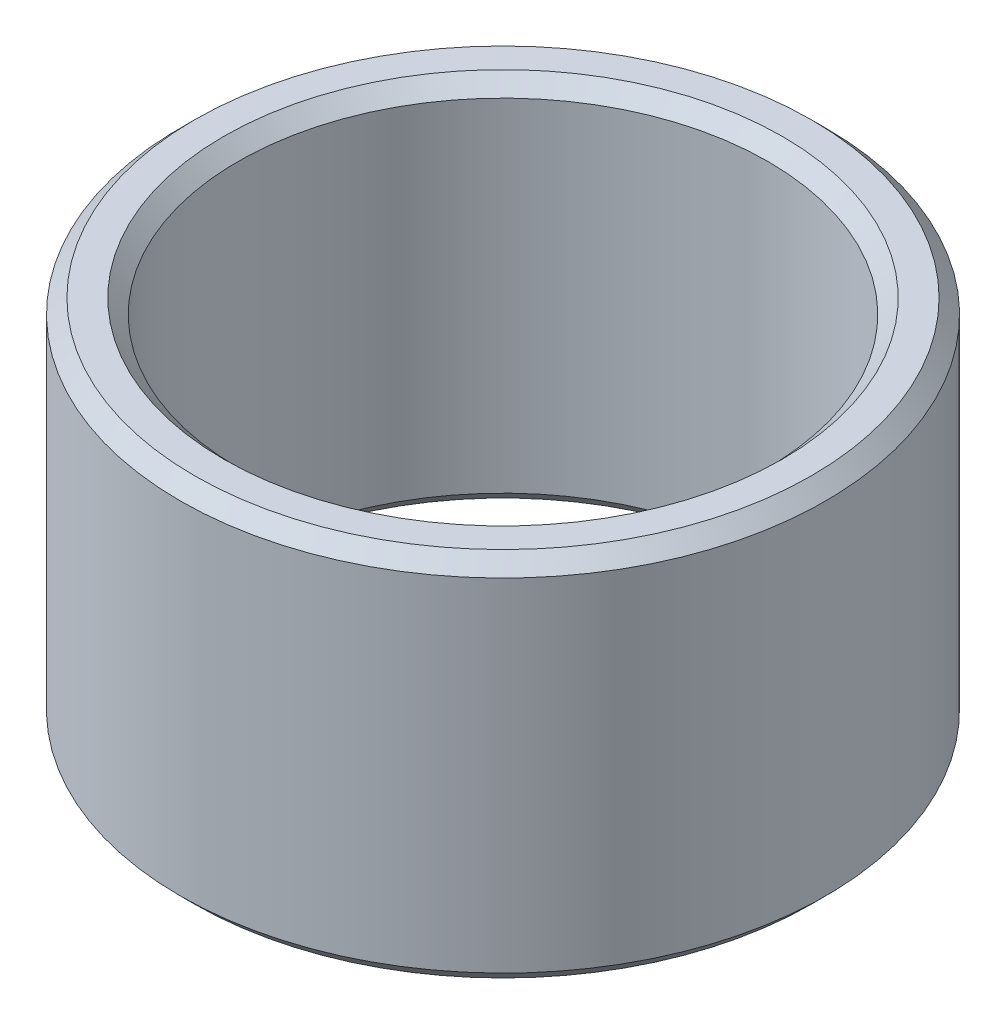
SolidWorks part; units mm, degrees
material "普通碳钢"
ref_plane "Front Plane" through (0, 0, 0) normal (0, 0, 1) x (1, 0, 0)
ref_plane "Top Plane" through (0, 0, 0) normal (0, 1, 0) x (1, 0, 0)
ref_plane "Right Plane" through (0, 0, 0) normal (1, 0, 0) x (0, 0, -1)
sketch "Sketch1" plane through (0, 0, 0) normal (0, 1, 0) x (1, 0, 0)
  circle A0 centre (0, 0) radius 33.5
  circle A1 centre (0, 0) radius 27.5
  dimension "D1" = 67
  dimension "D2" = 55
extrude "Boss-Extrude1" add sketch "Sketch1" along normal blind 38.5
chamfer "Chamfer1" distance 1.5 angle 45 4 edges at (0, 0, 27.5) (0, 0, 33.5) (0, 38.5, 27.5) (0, 38.5, 33.5)
